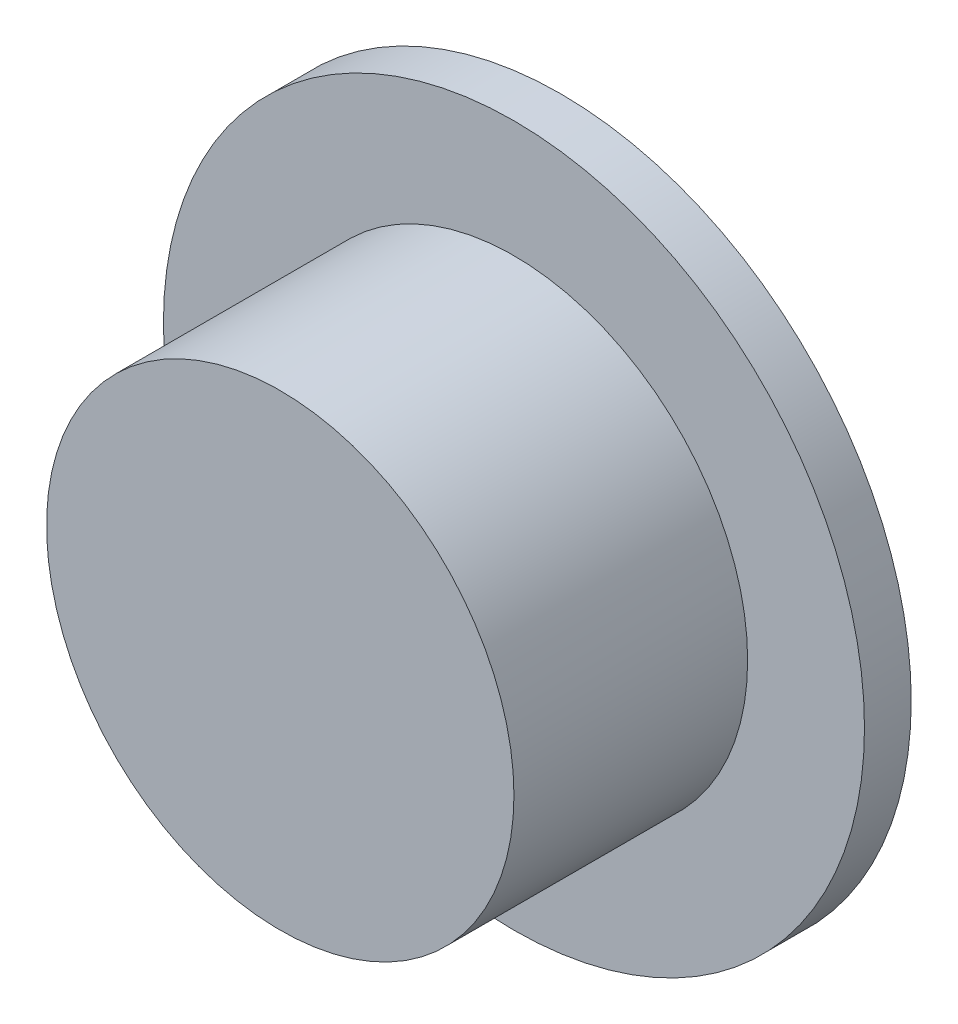
from build123d import *

# Parameters (mm, degrees)
SKETCH1_R           = 15
BOSS_EXTRUDE1_DEPTH = 2
SKETCH2_R           = 10
BOSS_EXTRUDE2_DEPTH = 10


with BuildPart() as part:
    # Sketch1 → Boss-Extrude1 (new body)
    with BuildSketch(Plane.XY):
        Circle(SKETCH1_R)
    extrude(amount=BOSS_EXTRUDE1_DEPTH)

    # Sketch2 → Boss-Extrude2 (add)
    with BuildSketch(Plane.XY.offset(2)):
        Circle(SKETCH2_R)
    extrude(amount=BOSS_EXTRUDE2_DEPTH)


solid = part.part
